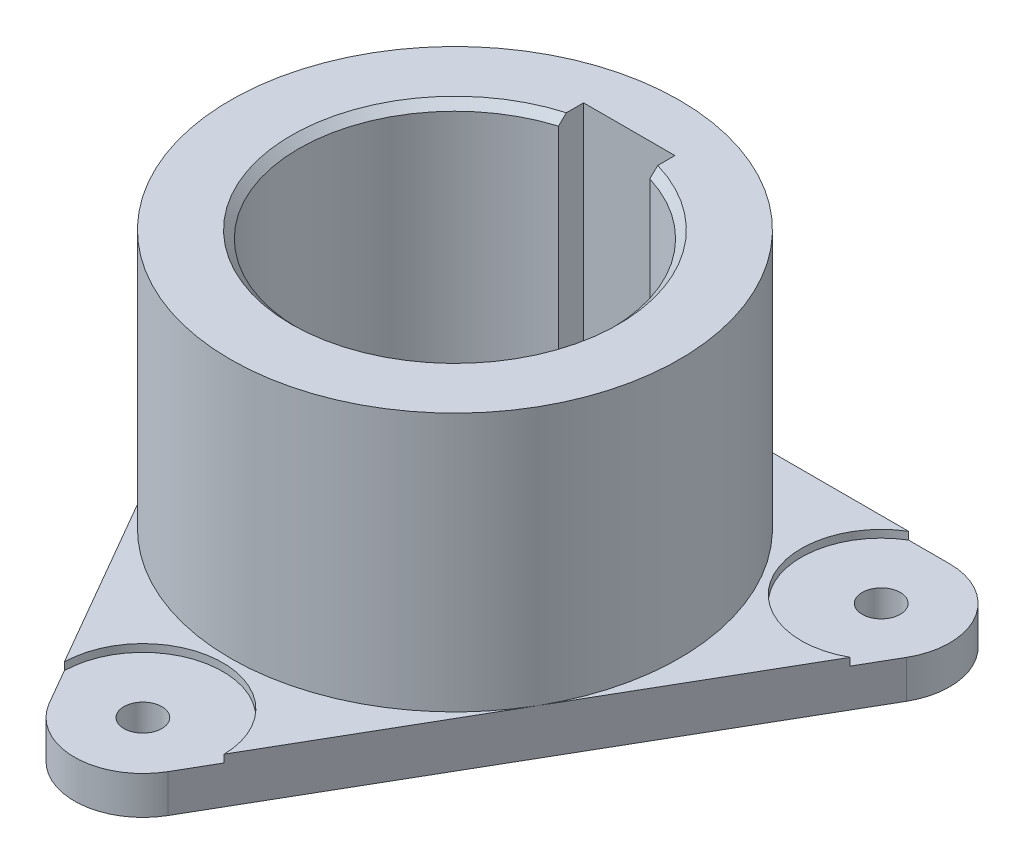
from build123d import *

# Parameters (mm, degrees)
EXTRUDE_1_DEPTH        = 6
EXTRUDE_1_2_DEPTH      = 6
EXTRUDE_1_3_DEPTH      = 6
SKETCH_2_R             = 29.5
EXTRUDE_2_DEPTH        = 40
CHAMFER_1_SIZE         = 1
HOLE_WIZARD_M6_1_D     = 5
HOLE_WIZARD_M6_1_DEPTH = 15
HOLE_WIZARD_M6_1_TIP   = 1.502151548
SKETCH_5_R             = 10.5
CUT_EXTRUDE_1_DEPTH    = 1


with BuildPart() as part:
    # 草图1 → 凸台-拉伸1 (new body)
    with BuildSketch(Plane(origin=(0, 0, 0), x_dir=(1, 0, 0), z_dir=(0, 1, 0))):
        with BuildLine():
            Line((1.03e-07, 29.5), (-35.507041555, 29.5))
            ThreePointArc((-35.507041555, 29.5), (-43.301270189, 25), (-43.301270189, 16))
            Line((-43.301270189, 16), (-25.547749424, -14.749999978))
            ThreePointArc((-25.547749424, -14.749999978), (-25.54774938, 14.750000056), (1.03e-07, 29.5))
        make_face()
    extrude(amount=EXTRUDE_1_DEPTH)



with BuildPart() as body_2:
    # 草图1 → Extrude 1 2 (new body)
    with BuildSketch(Plane(origin=(0, 0, 0), x_dir=(1, 0, 0), z_dir=(0, 1, 0))):
        with BuildLine():
            ThreePointArc((25.547749421, -14.749999984), (-3e-09, -29.5), (-25.547749424, -14.749999978))
            Line((-25.547749424, -14.749999978), (-7.794228634, -45.5))
            ThreePointArc((-7.794228634, -45.5), (0, -50), (7.794228634, -45.5))
            Line((7.794228634, -45.5), (25.547749421, -14.749999984))
        make_face()
    extrude(amount=EXTRUDE_1_2_DEPTH)


with BuildPart() as body_3:
    # 草图1 → Extrude 1 3 (new body)
    with BuildSketch(Plane(origin=(0, 0, 0), x_dir=(1, 0, 0), z_dir=(0, 1, 0))):
        with BuildLine():
            Line((35.507041555, 29.5), (1.03e-07, 29.5))
            ThreePointArc((1.03e-07, 29.5), (20.859650082, 20.859650009), (29.5, 0))
            ThreePointArc((29.5, 0), (28.494811878, -7.635161822), (25.547749421, -14.749999984))
            Line((25.547749421, -14.749999984), (43.301270189, 16))
            ThreePointArc((43.301270189, 16), (43.301270189, 25), (35.507041555, 29.5))
        make_face()
    extrude(amount=EXTRUDE_1_3_DEPTH)


with BuildPart() as part_1:
    add(part.part)

    add(body_2.part)  # 凸台-拉伸2 merges body 2

    add(body_3.part)  # 凸台-拉伸2 merges body 3
    # 草图2 → 凸台-拉伸2 (add)
    with BuildSketch(Plane(origin=(0, 0, 0), x_dir=(1, 0, 0), z_dir=(0, 1, 0))):
        with Locations(Location((0, 0, 0), (0, 0, 90))):
            Circle(SKETCH_2_R)
        with BuildLine():
            Line((6, 19.602295784), (6, 22.902295784))
            Line((6, 22.902295784), (-6, 22.902295784))
            Line((-6, 22.902295784), (-6, 19.602295784))
            ThreePointArc((-6, 19.602295784), (0, -20.5), (6, 19.602295784))
        make_face(mode=Mode.SUBTRACT)
    extrude(amount=EXTRUDE_2_DEPTH)

    # 倒角1
    chamfer_1_edges = [part_1.edges().sort_by_distance(p)[0] for p in [
        (0, 0, 20.5),
        (0, 40, 20.5),
    ]]
    chamfer(chamfer_1_edges, length=CHAMFER_1_SIZE)

    # M6 螺纹孔1
    with Locations(Plane(origin=(0, 6, 0), x_dir=(1, 0, 0), z_dir=(0, 1, 0))):
        with Locations((-35.507041555, 20.5), (35.507041555, 20.5), (0, -41)):
            Hole(HOLE_WIZARD_M6_1_D / 2, depth=HOLE_WIZARD_M6_1_DEPTH)
            with Locations((0, 0, -(HOLE_WIZARD_M6_1_DEPTH + HOLE_WIZARD_M6_1_TIP / 2))):  # 118° drill point
                Cone(0, HOLE_WIZARD_M6_1_D / 2, HOLE_WIZARD_M6_1_TIP, mode=Mode.SUBTRACT)

    # 草图5 → 切除-拉伸1 (cut)
    with BuildSketch(Plane(origin=(0, 6, 0), x_dir=(1, 0, 0), z_dir=(0, 1, 0))):
        with Locations((-35.507041555, 20.5)):
            Circle(SKETCH_5_R)
        with Locations((35.507041555, 20.5)):
            Circle(SKETCH_5_R)
        with Locations((0, -41)):
            Circle(SKETCH_5_R)
    extrude(amount=-CUT_EXTRUDE_1_DEPTH, mode=Mode.SUBTRACT)


solid = part_1.part
